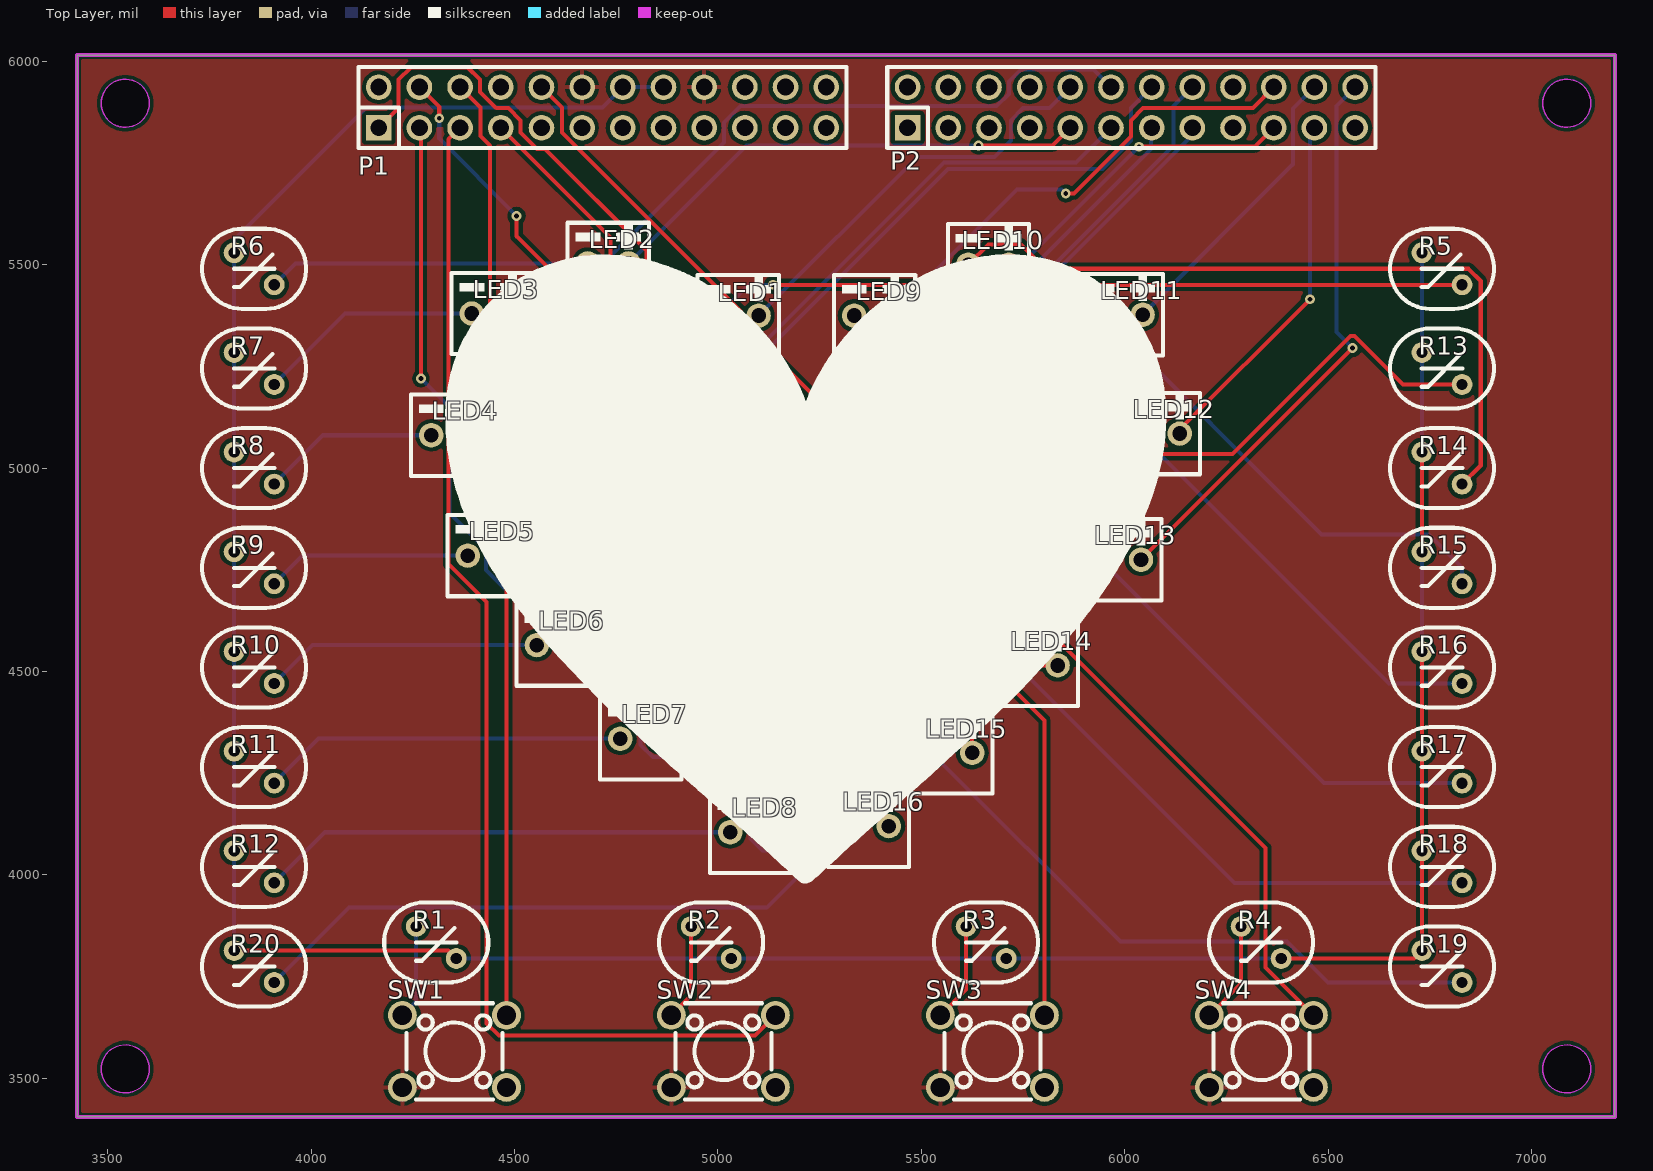
[diagram p0: Top Layer view]
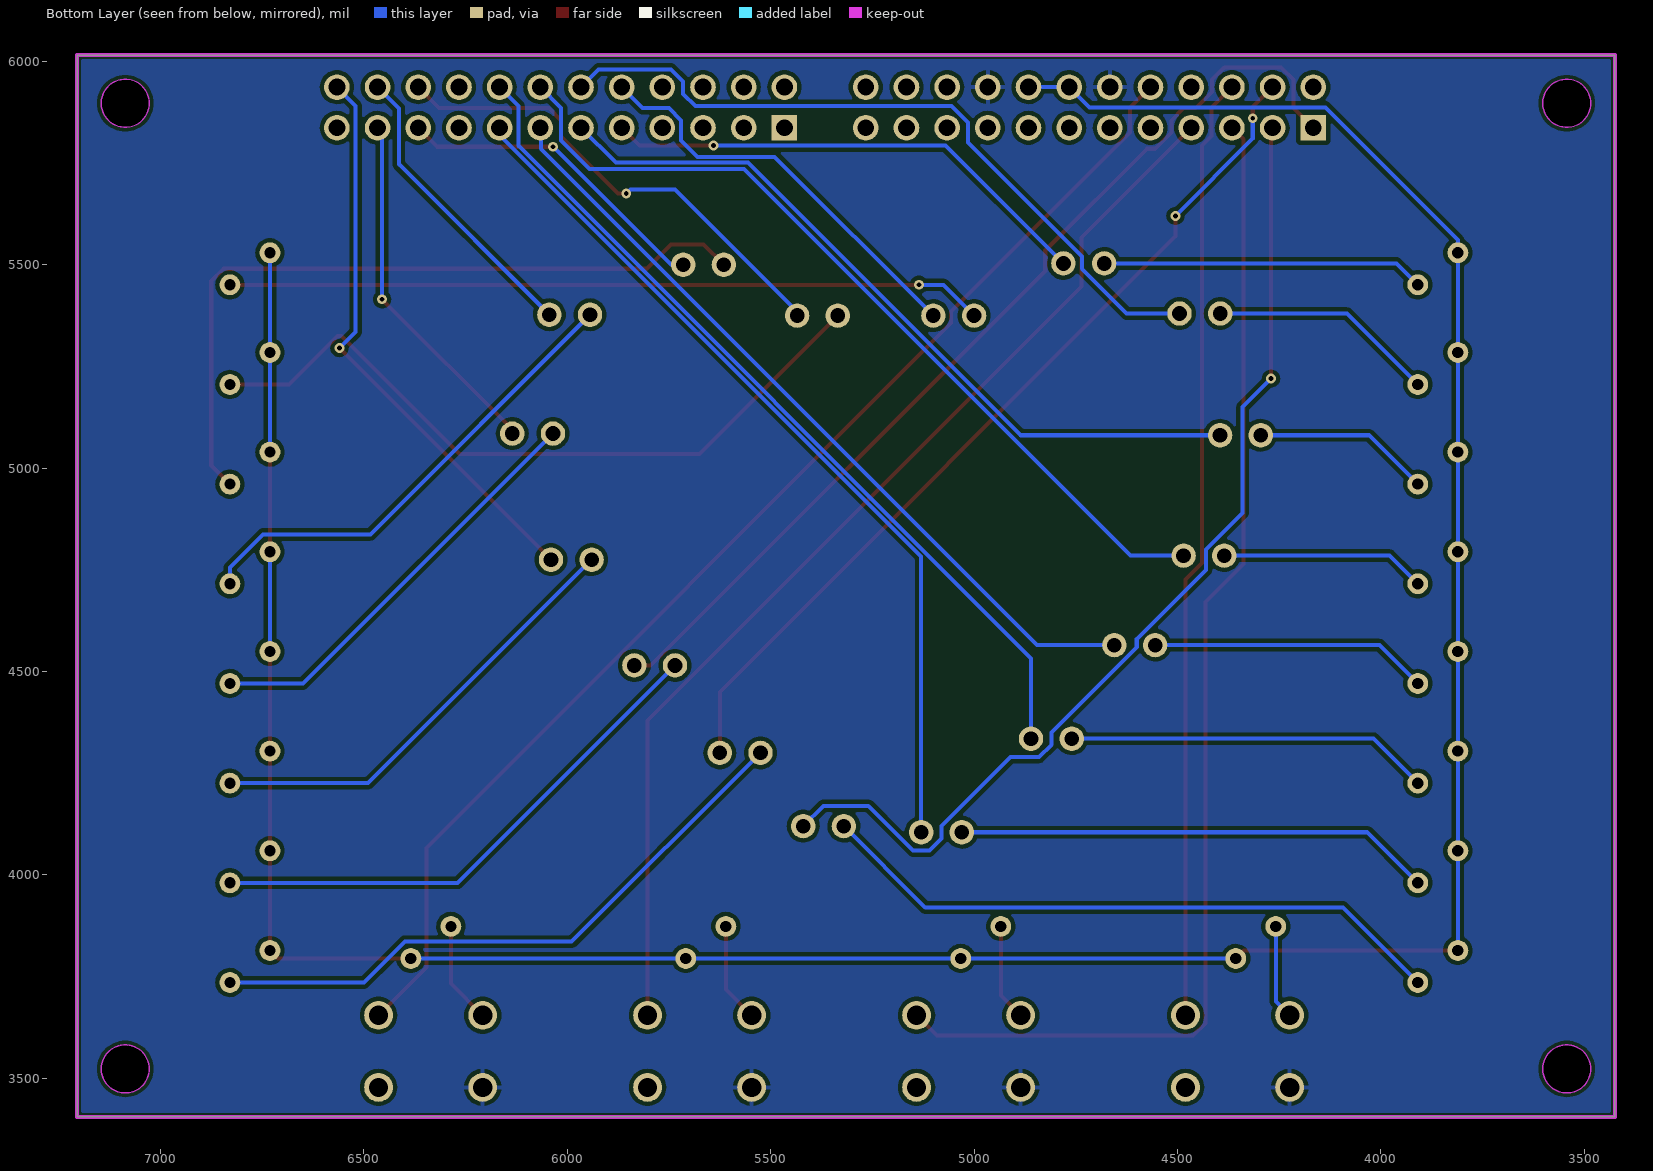
[diagram p1: Bottom Layer view, seen from below]
# Altium PCB MISC51818.pcbdoc
Units mil, origin at the board's own origin, x right, y up, seen from the top; angles counter-clockwise.
Board outline 3779.53 x 2609.84 mil, 2 copper layers (Top Layer, Bottom Layer), stack 62.206 mil thick; 42 components, 66 nets, 136 pads, 9 vias.

## Layer stack, top to bottom
Top Solder Mask Layer: solder mask 0.394, Dk 3.3
Top Layer: signal copper 1.379
Dielectric1: surface 59.449, FR4, Dk 4.5
Bottom Layer: signal copper 1.378
Bottom Solder Mask Layer: solder mask 0.394, Dk 3.3

## Board outline
3425,6015 3425,3405.16 7204.53,3405.16 7204.53,6015
cut-out: 3602.17,5896.89 cw(c3543.11,5896.89) 3484.06,5896.89 cw(c3543.11,5896.89)
cut-out: 3602.17,3523.27 cw(c3543.11,3523.27) 3484.06,3523.27 cw(c3543.11,3523.27)
cut-out: 7145.47,3523.27 cw(c7086.42,3523.27) 7027.36,3523.27 cw(c7086.42,3523.27)
cut-out: 7145.47,5896.89 cw(c7086.42,5896.89) 7027.36,5896.89 cw(c7086.42,5896.89)

## Design rules (kind name [scope] priority, off if disabled: settings)
BoardOutlineClearance copperThickness2oz_1 [All] p2 off: genericclearance=7.99 ignorepadtopadclearanceinfootprint=FALSE except(0: Arc-SplitContinuation Track-SplitContinuation SMDPad-SplitContinuation THPad-SplitContinuation Via-SplitContinuation Fill-SplitContinuation Region-SplitContinuation Poly-SplitContinuation Text-SplitContinuation Hole-SplitContinuation; 5.98: Arc-CutoutEdge SMDPad-CutoutEdge THPad-CutoutEdge Via-CutoutEdge Fill-CutoutEdge Region-CutoutEdge Text-CutoutEdge; 6.93: Hole-OutlineEdge Hole-CutoutEdge; 10: Poly-OutlineEdge Poly-CutoutEdge; 11.81: Arc-OutlineEdge Track-OutlineEdge SMDPad-OutlineEdge THPad-OutlineEdge Via-OutlineEdge Fill-OutlineEdge Region-OutlineEdge Text-OutlineEdge Track-CutoutEdge)
BoardOutlineClearance Plane_innerPlane_1 [All] p4 off: genericclearance=4.02 ignorepadtopadclearanceinfootprint=FALSE except(0: Arc-SplitContinuation Track-SplitContinuation SMDPad-SplitContinuation THPad-SplitContinuation Via-SplitContinuation Fill-SplitContinuation Region-SplitContinuation Poly-SplitContinuation Text-SplitContinuation Hole-SplitContinuation; 6: SMDPad-CutoutEdge THPad-CutoutEdge Via-CutoutEdge Fill-CutoutEdge Region-CutoutEdge Text-CutoutEdge; 6.93: Hole-OutlineEdge Hole-CutoutEdge; 10: Poly-OutlineEdge Poly-CutoutEdge; 11.8: Arc-OutlineEdge Track-OutlineEdge SMDPad-OutlineEdge THPad-OutlineEdge Via-OutlineEdge Fill-OutlineEdge Region-OutlineEdge Text-OutlineEdge; 11.81: Arc-CutoutEdge Track-CutoutEdge)
BoardOutlineClearance Copper_copperRegion_1 [All] p6 off: genericclearance=4.02 ignorepadtopadclearanceinfootprint=FALSE except(0: Arc-SplitContinuation Track-SplitContinuation SMDPad-SplitContinuation THPad-SplitContinuation Via-SplitContinuation Fill-SplitContinuation Region-SplitContinuation Poly-SplitContinuation Text-SplitContinuation Hole-SplitContinuation; 6: SMDPad-CutoutEdge THPad-CutoutEdge Via-CutoutEdge Fill-CutoutEdge Region-CutoutEdge Text-CutoutEdge; 6.93: Hole-OutlineEdge Hole-CutoutEdge; 10: Poly-OutlineEdge Poly-CutoutEdge; 11.8: Arc-OutlineEdge Track-OutlineEdge SMDPad-OutlineEdge THPad-OutlineEdge Via-OutlineEdge Fill-OutlineEdge Region-OutlineEdge Text-OutlineEdge; 11.81: Arc-CutoutEdge Track-CutoutEdge)
BoardOutlineClearance copperThickness1oz_1 [All] p8: genericclearance=4.02 ignorepadtopadclearanceinfootprint=FALSE except(0: Arc-SplitContinuation Track-SplitContinuation SMDPad-SplitContinuation THPad-SplitContinuation Via-SplitContinuation Fill-SplitContinuation Region-SplitContinuation Poly-SplitContinuation Text-SplitContinuation Hole-SplitContinuation; 6: SMDPad-CutoutEdge THPad-CutoutEdge Via-CutoutEdge Fill-CutoutEdge Region-CutoutEdge Text-CutoutEdge; 6.93: Hole-OutlineEdge Hole-CutoutEdge; 10: Poly-OutlineEdge Poly-CutoutEdge; 11.8: Arc-OutlineEdge Track-OutlineEdge SMDPad-OutlineEdge THPad-OutlineEdge Via-OutlineEdge Fill-OutlineEdge Region-OutlineEdge Text-OutlineEdge; 11.81: Arc-CutoutEdge Track-CutoutEdge)
Clearance copperThickness2oz [All] p1 off: gap=7.99 ignorepadtopadclearanceinfootprint=FALSE except(5.98: SMDPad-Track SMDPad-SMDPad THPad-Track SMDPad-THPad THPad-THPad Track-Via SMDPad-Via THPad-Via Via-Via Fill-Track Region-Track Fill-SMDPad Region-SMDPad Fill-THPad Region-THPad Fill-Via Region-Via Fill-Fill Fill-Region Region-Region Arc-Track Arc-SMDPad Arc-THPad Arc-Via Fill-Arc Region-Arc Arc-Arc Text-Track SMDPad-Text Text-THPad Text-Via Fill-Text Region-Text Arc-Text Text-Text; 6.93: Hole-Track Hole-SMDPad Hole-THPad Hole-Via Fill-Hole Region-Hole Hole-Arc Hole-Text; 10: Poly-Track Poly-SMDPad Poly-THPad Poly-Via Poly-Fill Poly-Region Poly-Poly Poly-Arc Poly-Text Poly-Hole)
Clearance Plane_innerPlane [All] p3 off: gap=4.02 ignorepadtopadclearanceinfootprint=FALSE except(5.98: SMDPad-Track SMDPad-SMDPad THPad-Track SMDPad-THPad THPad-THPad Track-Via SMDPad-Via THPad-Via Via-Via Fill-Track Region-Track Fill-SMDPad Region-SMDPad Fill-THPad Region-THPad Fill-Via Region-Via Fill-Fill Fill-Region Region-Region; 6: Arc-Track Arc-SMDPad Arc-THPad Arc-Via Fill-Arc Region-Arc Arc-Arc Text-Track SMDPad-Text Text-THPad Text-Via Fill-Text Region-Text Arc-Text Text-Text; 6.93: Hole-Track Hole-SMDPad Hole-THPad Hole-Via Fill-Hole Region-Hole Hole-Arc Hole-Text; 10: Poly-Track Poly-SMDPad Poly-THPad Poly-Via Poly-Fill Poly-Region Poly-Poly Poly-Arc Poly-Text Poly-Hole)
Clearance Copper_copperRegion [All] p5 off: gap=4.02 ignorepadtopadclearanceinfootprint=FALSE except(5.98: SMDPad-Track SMDPad-SMDPad THPad-Track SMDPad-THPad THPad-THPad Track-Via SMDPad-Via THPad-Via Via-Via Fill-Track Region-Track Fill-SMDPad Region-SMDPad Fill-THPad Region-THPad Fill-Via Region-Via Fill-Fill Fill-Region Region-Region; 6: Arc-Track Arc-SMDPad Arc-THPad Arc-Via Fill-Arc Region-Arc Arc-Arc Text-Track SMDPad-Text Text-THPad Text-Via Fill-Text Region-Text Arc-Text Text-Text; 6.93: Hole-Track Hole-SMDPad Hole-THPad Hole-Via Fill-Hole Region-Hole Hole-Arc Hole-Text; 10: Poly-Track Poly-SMDPad Poly-THPad Poly-Via Poly-Fill Poly-Region Poly-Poly Poly-Arc Poly-Text Poly-Hole)
Clearance copperThickness1oz [All] p7: gap=4.02 ignorepadtopadclearanceinfootprint=FALSE except(5.98: SMDPad-Track SMDPad-SMDPad THPad-Track SMDPad-THPad THPad-THPad Track-Via SMDPad-Via THPad-Via Via-Via Fill-Track Region-Track Fill-SMDPad Region-SMDPad Fill-THPad Region-THPad Fill-Via Region-Via Fill-Fill Fill-Region Region-Region; 6: Arc-Track Arc-SMDPad Arc-THPad Arc-Via Fill-Arc Region-Arc Arc-Arc Text-Track SMDPad-Text Text-THPad Text-Via Fill-Text Region-Text Arc-Text Text-Text; 6.93: Hole-Track Hole-SMDPad Hole-THPad Hole-Via Fill-Hole Region-Hole Hole-Arc Hole-Text; 10: Poly-Track Poly-SMDPad Poly-THPad Poly-Via Poly-Fill Poly-Region Poly-Poly Poly-Arc Poly-Text Poly-Hole)
DiffPairsRouting differentialPair [All] p1: maxlimit=6 minlimit=6 mostfreqgap=6 toplayer_minwidth=5 toplayer_prefwidth=10 toplayer_maxwidth=100 toplayer_mingap=6 toplayer_prefgap=6 toplayer_maxgap=6 bottomlayer_minwidth=5 bottomlayer_prefwidth=10 bottomlayer_maxwidth=100 bottomlayer_mingap=6 bottomlayer_prefgap=6 bottomlayer_maxgap=6 maxuncoupledlength=10
HoleToHoleClearance otherClearance [All] p1: gap=11.81 allowstackedmicrovias=TRUE
Length netLength [All] p1: minlimit=0 maxlimit=0
PasteMaskExpansion pasteMaskExpansion [All] p1: expansion=0
PlaneConnect innerPlane [All] p1: planeconnectstyle=Relief reliefexpansion=20 reliefentries=4 reliefconductorwidth=10 reliefairgap=10
PolygonConnect copperRegion [All] p1: connectstyle=Relief reliefconductorwidth=10 reliefentries=4 polygonreliefangle="90 Angle" airgapwidth=10 via.connectstyle=Relief via.reliefconductorwidth=10 via.reliefentries=4 via.polygonreliefangle="90 Angle" via.airgapwidth=10
RoutingVias viaSize [All] p1: holewidth=12.01 width=24.02 viastyle="Through Hole" minholewidth=11.81 minwidth=19.68 maxholewidth=248.03 maxwidth=393.7
SolderMaskExpansion solderMaskExpansion [IsVia] p1: expansion=-1000 istentingtop=TRUE
SolderMaskExpansion solderMaskExpansion [All] p2: expansion=2 istentingtop=FALSE
Width copperThickness2oz_2 [All] p1 off: maxlimit=100 minlimit=8 preferedwidth=10
Width copperThickness1oz_2 [All] p2: maxlimit=100 minlimit=5 preferedwidth=10

## Components (designator, comment, footprint, x,y, rotation, side; value= is the part's Value field where it differs from the comment)
LED1 "" LED-TH_L5.0-W5.0-P2.54_RED 5050,5375 r180 top
LED2 "" LED-TH_L5.0-W5.0-P2.54_RED 4730.3,5503.15 r180 top
LED3 "" LED-TH_L5.0-W5.0-P2.54_RED 4445,5380 r180 top
LED4 "" LED-TH_L5.0-W5.0-P2.54_RED 4345.3,5080.86 r180 top
LED5 "" LED-TH_L5.0-W5.0-P2.54_RED 4435,4785 r180 top
LED6 "" LED-TH_L5.0-W5.0-P2.54_RED 4605,4565 r180 top
LED7 "" LED-TH_L5.0-W5.0-P2.54_RED 4810,4335 r180 top
LED8 "" LED-TH_L5.0-W5.0-P2.54_RED 5080,4105 r180 top
LED9 "" LED-TH_L5.0-W5.0-P2.54_RED 5385,5375 r180 top
LED10 "" LED-TH_L5.0-W5.0-P2.54_RED 5665,5500 r180 top
LED11 "" LED-TH_L5.0-W5.0-P2.54_RED 5993.93,5377 r180 top
LED12 "" LED-TH_L5.0-W5.0-P2.54_RED 6085,5085 r180 top
LED13 "" LED-TH_L5.0-W5.0-P2.54_RED 5990,4775 r180 top
LED14 "" LED-TH_L5.0-W5.0-P2.54_RED 5785,4515 r180 top
LED15 "" LED-TH_L5.0-W5.0-P2.54_RED 5575,4300 r180 top
LED16 "" LED-TH_L5.0-W5.0-P2.54_RED 5370,4120 r180 top
P1 "2.54-2*12P female" HDR-TH_24P-P2.54-V-F-R2-C12-S2.54 4716.19,5886.46 r0 top
P2 "2.54-2*12P female" HDR-TH_24P-P2.54-V-F-R2-C12-S2.54 6016.19,5886.46 r0 top
R1 "4.7K" RES-TH_RES-TH_L6.5-W5.0-P2.50-D0.4-S2.00 4307.53,3834.14 r0 top
R2 "4.7K" RES-TH_RES-TH_L6.5-W5.0-P2.50-D0.4-S2.00 4983.42,3834.14 r0 top
R3 "4.7K" RES-TH_RES-TH_L6.5-W5.0-P2.50-D0.4-S2.00 5659.31,3834.14 r0 top
R4 "4.7K" RES-TH_RES-TH_L6.5-W5.0-P2.50-D0.4-S2.00 6335.2,3834.14 r0 top
R5 "1K" RES-TH_RES-TH_L6.5-W5.0-P2.50-D0.4-S2.00 6780,5490 r0 top
R6 "1K" RES-TH_RES-TH_L6.5-W5.0-P2.50-D0.4-S2.00 3860,5490 r0 top
R7 "1K" RES-TH_RES-TH_L6.5-W5.0-P2.50-D0.4-S2.00 3860,5245 r0 top
R8 "1K" RES-TH_RES-TH_L6.5-W5.0-P2.50-D0.4-S2.00 3860,5000 r0 top
R9 "1K" RES-TH_RES-TH_L6.5-W5.0-P2.50-D0.4-S2.00 3860,4755 r0 top
R10 "1K" RES-TH_RES-TH_L6.5-W5.0-P2.50-D0.4-S2.00 3860,4510 r0 top
R11 "1K" RES-TH_RES-TH_L6.5-W5.0-P2.50-D0.4-S2.00 3860,4265 r0 top
R12 "1K" RES-TH_RES-TH_L6.5-W5.0-P2.50-D0.4-S2.00 3860,4020 r0 top
R13 "1K" RES-TH_RES-TH_L6.5-W5.0-P2.50-D0.4-S2.00 6780,5245 r0 top
R14 "1K" RES-TH_RES-TH_L6.5-W5.0-P2.50-D0.4-S2.00 6780,5000 r0 top
R15 "1K" RES-TH_RES-TH_L6.5-W5.0-P2.50-D0.4-S2.00 6780,4755 r0 top
R16 "1K" RES-TH_RES-TH_L6.5-W5.0-P2.50-D0.4-S2.00 6780,4510 r0 top
R17 "1K" RES-TH_RES-TH_L6.5-W5.0-P2.50-D0.4-S2.00 6780,4265 r0 top
R18 "1K" RES-TH_RES-TH_L6.5-W5.0-P2.50-D0.4-S2.00 6780,4020 r0 top
R19 "1K" RES-TH_RES-TH_L6.5-W5.0-P2.50-D0.4-S2.00 6780,3775 r0 top
R20 "1K" RES-TH_RES-TH_L6.5-W5.0-P2.50-D0.4-S2.00 3860,3775 r0 top
SW1 "TS665CJ" SW-TH_4P-L6.0-W6.0-P4.50-LS6.5 4352.21,3566.44 r0 top
SW2 "TS665CJ" SW-TH_4P-L6.0-W6.0-P4.50-LS6.5 5013.41,3566.44 r0 top
SW3 "TS665CJ" SW-TH_4P-L6.0-W6.0-P4.50-LS6.5 5674.6,3566.44 r0 top
SW4 "TS665CJ" SW-TH_4P-L6.0-W6.0-P4.50-LS6.5 6335.8,3566.44 r0 top

## Footprints (in the part's own frame and the unit in brackets; to place one, negate y for a bottom-side part, rotate by r counter-clockwise, add the part's x,y. Pads: shape width x height; smd on the part's side, far side on the other; paste and mask are expansions set on the pad)
HDR-TH_24P-P2.54-V-F-R2-C12-S2.54 [mm]
  rect 1.6x1.6 hole 1.05: 1(-13.97,-1.27)
  round 1.6 hole 1.05: 2(-13.97,1.27) 3(-11.43,-1.27) 4(-11.43,1.27) 5(-8.89,-1.27) 6(-8.89,1.27) 7(-6.35,-1.27) 8(-6.35,1.27) 9(-3.81,-1.27) 10(-3.81,1.27) 11(-1.27,-1.27) 12(-1.27,1.27) 13(1.27,-1.27) 14(1.27,1.27) 15(3.81,-1.27) 16(3.81,1.27) 17(6.35,-1.27) 18(6.35,1.27) 19(8.89,-1.27) 20(8.89,1.27) 21(11.43,-1.27) 22(11.43,1.27) 23(13.97,-1.27) 24(13.97,1.27)
  silkscreen extent -15.24,-2.54 15.24,2.54
LED-TH_L5.0-W5.0-P2.54_RED [mil]
  round 60 hole 36 paste+0 mask+1.97: 1(-50,0) 2(50,0)
  silkscreen extent -100,-100 100,100
RES-TH_RES-TH_L6.5-W5.0-P2.50-D0.4-S2.00 [mm]
  round 1.3 hole 0.7: 1(-1.25,1) 2(1.25,-1)
  silkscreen extent -3.25,-2.5 3.25,2.5
SW-TH_4P-L6.0-W6.0-P4.50-LS6.5 [mm]
  round 1.8 hole 1.2: 1(-3.25,2.25) 2(3.25,2.25) 3(-3.25,-2.25) 4(3.25,-2.25)
  silkscreen extent -3,-3 3,3

## Via types
v1: diameter 24.02, hole 12, Top Layer to Bottom Layer, 9 vias

## Nets (pads, with @x,y where several pads share a name; then routed paths per layer and width w, separated by ;. In a path a pad name is that pad's centre, name@x,y a point inside that pad or via, vN(x,y) a via of type N, cw(c..) or ccw(c..) an arc to the next point about the centre after c; other vN are vias at no path point)
$1N1: R1.1 SW1.1 | length 232.6
  Bottom Layer w10: SW1.1 4258.32,3689.07 R1.1
$1N8: R2.1 SW2.1 | length 238.7
  Top Layer w10: SW2.1 4934.21,3703.77 R2.1
$1N12: R3.1 SW3.1 | length 244.8
  Top Layer w10: SW3.1 5610.1,3718.46 R3.1
$1N16: R4.1 SW4.1 | length 250.9
  Top Layer w10: SW4.1@6207.86,3655.01 6285.99,3733.15 R4.1
$1N17: LED1.2 R5.2 | length 1860.5
  Top Layer w10: v1(5135.63,5450.63) R5.2
  Bottom Layer w10: LED1.2 5075.63,5450.63 v1(5135.63,5450.63)
$1N18: LED2.2 R6.2 | length 792.8
  Bottom Layer w10: R6.2 3961.73,5503.15 LED2.2
$1N19: LED3.2 R7.2 | length 558
  Bottom Layer w10: R7.2 4083.58,5380 LED3.2
$1N20: LED4.2 R8.2 | length 435.9
  Bottom Layer w10: R8.2 4029.44,5080.86 LED4.2
$1N21: LED5.2 R9.2 | length 504.5
  Bottom Layer w10: R9.2 3978.58,4785 LED5.2
$1N22: LED8.2 R12.2 | length 1172.3
  Bottom Layer w10: R12.2 4033.58,4105 LED8.2
$1N23: LED6.2 R10.2 | length 684.9
  Bottom Layer w10: R10.2 4003.58,4565 LED6.2
$1N24: LED7.2 R11.2 | length 896.1
  Bottom Layer w10: R11.2 4018.58,4335 LED7.2
$1N25: LED9.2 R13.2 | length 1804.6
  Top Layer w10: LED9.2 5675,5035 6265,5035 6555,5325 6565,5325 6684.37,5205.63 R13.2
$1N26: LED13.2 R17.2 | length 1116.8
  Bottom Layer w10: LED13.2 6489.37,4225.63 R17.2
$1N27: LED12.2 R16.2 | length 1048.7
  Bottom Layer w10: LED12.2 6649.37,4470.63 R16.2
$1N28: LED11.2 R15.2 | length 1182.7
  Bottom Layer w10: LED11.2 6483.93,4837 6747.84,4837 6829.21,4755.63 R15.2
$1N29: LED14.2 R18.2 | length 1315.6
  Bottom Layer w10: LED14.2 6269.37,3980.63 R18.2
$1N30: LED10.2 R14.2 | length 1836.3
  Top Layer w10: LED10.2 5665,5550 5745,5550 5805,5490 6845,5490 6875,5460 6875,5006.41 R14.2
$1N31: LED16.2 R20.2 | length 1570
  Bottom Layer w10: R20.2 4093.58,3920 5120,3920 LED16.2
$1N32: LED15.2 R19.2 | length 1538
  Bottom Layer w10: LED15.2 5989.01,3835.99 6399.01,3835.99 6499.37,3735.63 R19.2
GND: P1.12 P1.18 SW1.3 SW2.3 SW3.3 SW4.3
P00: LED9.1 P2.20 | length 1201.3
  Top Layer w10: v1(5855,5675) 5875,5675 6015,5815 6015,5855 6045,5885 6314.72,5885 P2.20
  Bottom Layer w10: LED9.1 5435,5385 5735,5685 5845,5685 v1(5855,5675)
P01: LED10.1 P2.19 | length 790.6
  Top Layer w10: v1(6035,5790) 6319.72,5790 P2.19
  Bottom Layer w10: LED10.1 5745,5500 v1(6035,5790)
P02: LED11.1 P2.22 | length 734.4
  Bottom Layer w10: LED11.1 6413.93,5747 6413.93,5884.2 P2.22
P03: LED12.1 P2.21 | length 888.6
  Top Layer w10: LED12.1 6135,5095 v1(6455,5415)
  Bottom Layer w10: v1(6455,5415) 6455,5825.28 P2.21
P04: LED13.1 P2.24 | length 1412.6
  Top Layer w10: LED13.1 v1(6560,5295)
  Bottom Layer w10: v1(6560,5295) 6520,5335 6520,5890.28 P2.24
P05: LED14.1 P1.1 | length 2444.5
  Top Layer w10: P1.1 4215,5885.28 4215,5955 4245,5985 4385,5985 4415,5955 4415,5925 4455,5885 4485,5885 4515,5855 4515,5825 4555,5785 4575,5785 4825,5535 4825,5485 5795,4515 LED14.1
P06: LED15.1 P1.4 | length 2199.3
  Top Layer w10: P1.4 4315,5887.65 v1(4315,5860) ; v1(4505,5620) 4505,5570 5625,4450 LED15.1
  Bottom Layer w10: v1(4315,5860) 4315,5810 v1(4505,5620)
P07: LED16.1 P1.3 | length 2543.3
  Top Layer w10: P1.3 4270,5832.65 v1(4270,5220)
  Bottom Layer w10: v1(4270,5220) 4340,5150 4340,4890 4430,4800 4430,4750 4600,4580 4600,4560 4810,4350 4810,4320 4840,4290 4910,4290 5080,4120 5080,4090 5110,4060 5150,4060 5260,4170 5370,4170 LED16.1
P10: P1.6 SW1.2 | length 2328.7
  Top Layer w10: P1.6 4416.19,5886.46 4416.19,5816.46 4440.16,5792.49 4440.16,4766.46 4480.16,4726.47 SW1.2
P11: P1.5 SW2.2 | length 2994.8
  Top Layer w10: P1.5 4338.19,5808.47 4338.19,4764.46 4431.36,4671.3 4431.36,3635.01 4461.36,3605.01 5091.35,3605.01 SW2.2
P12: P1.7 SW3.2 | length 2735
  Top Layer w10: P1.7 4736.19,5566.46 4736.19,5446.46 5802.55,4380.1 SW3.2
P16: P1.10 SW4.2 | length 3067.4
  Top Layer w10: P1.10 4616.19,5886.46 4616.19,5825.1 5056.18,5385.11 5056.18,5356.46 6346.18,4066.47 6346.18,3772.59 SW4.2
P17: P1.9
P20: LED1.1 P2.10 | length 1028
  Bottom Layer w10: LED1.1 5490,5765 5680,5765 5720,5805 5720,5855 5750,5885 5814.72,5885 P2.10
P21: LED2.1 P2.9 | length 1224
  Top Layer w10: v1(5640.29,5793.15) 5822.87,5793.15 P2.9
  Bottom Layer w10: LED2.1 5070.3,5793.15 v1(5640.29,5793.15)
P22: LED3.1 P2.12 | length 1802.2
  Bottom Layer w10: LED3.1 4625,5380 4735,5490 4735,5520 5015,5800 5015,5850 5055,5890 5685,5890 5715,5920 5715,5950 5745,5980 5922.65,5980 P2.12
P23: LED4.1 P2.11 | length 1883.9
  Bottom Layer w10: LED4.1 4885.3,5080.86 5555.29,5750.86 5880.58,5750.86 P2.11
P24: LED5.1 P2.14 | length 2105.2
  Bottom Layer w10: LED5.1 4615,4785 5565,5735 5945,5735 6015,5805 6015,5885.27 P2.14
P25: LED6.1 P2.13 | length 1967.3
  Bottom Layer w10: LED6.1 4845,4565 6065,5785 6065,5835.27 P2.13
P26: LED7.1 P2.16 | length 2142.5
  Bottom Layer w10: LED7.1 4860,4532.48 6120,5792.48 6120,5890.27 P2.16
P27: LED8.1 P2.15 | length 2160.7
  Bottom Layer w10: LED8.1 5130,4782.48 6166.19,5818.67 P2.15
P32: P1.22
P33: P1.21
P34: P1.24
P35: P2.1
P40: P1.17
P41: P2.6
P42: P2.5
P43: P2.8
P44: P2.7
P45: P2.18
P46: P2.17
P47: P1.8
P50: P1.23
P51: P2.2
P52: P2.23
P53: P1.2
P54: P1.13
P55: P1.15
RXD-1: P1.20
RXD-2: P2.4
TXD-1: P1.19
TXD-2: P2.3
VCC: P1.14 P1.16 R1.2 R2.2 R3.2 R4.2 R5.1 R6.1 R7.1 R8.1 R9.1 R10.1 R11.1 R12.1 R13.1 R14.1 R15.1 R16.1 R17.1 R18.1 R19.1 R20.1 | length 7608.8
  Top Layer w10: R20.1 4337.15,3814.37 R1.2 ; R4.2 6711.19,3794.77 R19.1 R18.1 R17.1 R16.1 ; R15.1 R14.1
  Bottom Layer w10: R20.1 R12.1 R11.1 R10.1 R9.1 R8.1 R7.1 R6.1 3810.79,5561.06 4136.19,5886.46 4716.19,5886.46 P1.14 P1.16 ; R1.2 R2.2 R3.2 R4.2 ; R16.1 R15.1 ; R14.1 R13.1 R5.1
VREF: P1.11
pads on no net: SW1.4 SW2.4 SW3.4 SW4.4

## Polygon pours and split planes (outlines as drawn)
GND on Top Layer (solid, remove dead copper, pour order 0): 3000,6240 3000,3000 7965,3000 7965,6240
GND on Bottom Layer (solid, remove dead copper, pour order 2): 3130,6250 3130,3175 7785,3175 7785,6250

## Keep-outs
Board Outline Layer:
  region: 3602.17,5896.89 cw(c3543.11,5896.89) 3484.06,5896.89 cw(c3543.11,5896.89)
  circle w0.1: c3543.11,5896.89 r59.06
  region: 3602.17,5896.89 3601.77,5890.03 3600.57,5883.27 3598.6,5876.69 3595.88,5870.39 3592.45,5864.44 3588.35,5858.93 3583.64,5853.93 3578.38,5849.52 3572.64,5845.75 3566.5,5842.66 3560.05,5840.32 3553.36,5838.73 3546.54,5837.93 3539.68,5837.93 3532.86,5838.73 3526.17,5840.32 3519.72,5842.66 3513.58,5845.75 3507.84,5849.52 3502.58,5853.93 3497.87,5858.93 3493.77,5864.44 3490.34,5870.39 3487.62,5876.69 3485.65,5883.27 3484.45,5890.03 3484.06,5896.89 3484.45,5903.75 3485.65,5910.51 3487.62,5917.09 3490.34,5923.39 3493.77,5929.34 3497.87,5934.85 3502.58,5939.84 3507.84,5944.26 3513.58,5948.03 3519.72,5951.12 3526.17,5953.46 3532.86,5955.05 3539.68,5955.85 3546.54,5955.85 3553.36,5955.05 3560.05,5953.46 3566.5,5951.12 3572.64,5948.03 3578.38,5944.26 3583.64,5939.84 3588.35,5934.85 3592.45,5929.34 3595.88,5923.39 3598.6,5917.09 3600.57,5910.51 3601.77,5903.75
  region: 3602.17,3523.27 cw(c3543.11,3523.27) 3484.06,3523.27 cw(c3543.11,3523.27)
  circle w0.1: c3543.11,3523.27 r59.06
  region: 3602.17,3523.27 3601.77,3516.41 3600.57,3509.65 3598.6,3503.07 3595.88,3496.76 3592.45,3490.82 3588.35,3485.31 3583.64,3480.31 3578.38,3475.9 3572.64,3472.12 3566.5,3469.04 3560.05,3466.69 3553.36,3465.11 3546.54,3464.31 3539.68,3464.31 3532.86,3465.11 3526.17,3466.69 3519.72,3469.04 3513.58,3472.12 3507.84,3475.9 3502.58,3480.31 3497.87,3485.31 3493.77,3490.82 3490.34,3496.76 3487.62,3503.07 3485.65,3509.65 3484.45,3516.41 3484.06,3523.27 3484.45,3530.12 3485.65,3536.89 3487.62,3543.47 3490.34,3549.77 3493.77,3555.72 3497.87,3561.23 3502.58,3566.22 3507.84,3570.64 3513.58,3574.41 3519.72,3577.49 3526.17,3579.84 3532.86,3581.43 3539.68,3582.22 3546.54,3582.22 3553.36,3581.43 3560.05,3579.84 3566.5,3577.49 3572.64,3574.41 3578.38,3570.64 3583.64,3566.22 3588.35,3561.23 3592.45,3555.72 3595.88,3549.77 3598.6,3543.47 3600.57,3536.89 3601.77,3530.12
  region: 7145.47,3523.27 cw(c7086.42,3523.27) 7027.36,3523.27 cw(c7086.42,3523.27)
  circle w0.1: c7086.42,3523.27 r59.06
  region: 7145.47,3523.27 7145.07,3516.41 7143.88,3509.65 7141.91,3503.07 7139.19,3496.76 7135.76,3490.82 7131.66,3485.31 7126.94,3480.31 7121.68,3475.9 7115.94,3472.12 7109.81,3469.04 7103.35,3466.69 7096.67,3465.11 7089.85,3464.31 7082.98,3464.31 7076.16,3465.11 7069.48,3466.69 7063.03,3469.04 7056.89,3472.12 7051.15,3475.9 7045.89,3480.31 7041.18,3485.31 7037.08,3490.82 7033.64,3496.76 7030.92,3503.07 7028.95,3509.65 7027.76,3516.41 7027.36,3523.27 7027.76,3530.12 7028.95,3536.89 7030.92,3543.47 7033.64,3549.77 7037.08,3555.72 7041.18,3561.23 7045.89,3566.22 7051.15,3570.64 7056.89,3574.41 7063.03,3577.49 7069.48,3579.84 7076.16,3581.43 7082.98,3582.22 7089.85,3582.22 7096.67,3581.43 7103.35,3579.84 7109.81,3577.49 7115.94,3574.41 7121.68,3570.64 7126.94,3566.22 7131.66,3561.23 7135.76,3555.72 7139.19,3549.77 7141.91,3543.47 7143.88,3536.89 7145.07,3530.12
  region: 7145.47,5896.89 cw(c7086.42,5896.89) 7027.36,5896.89 cw(c7086.42,5896.89)
  circle w0.1: c7086.42,5896.89 r59.06
  region: 7145.47,5896.89 7145.07,5890.03 7143.88,5883.27 7141.91,5876.69 7139.19,5870.39 7135.76,5864.44 7131.66,5858.93 7126.94,5853.93 7121.68,5849.52 7115.94,5845.75 7109.81,5842.66 7103.35,5840.32 7096.67,5838.73 7089.85,5837.93 7082.98,5837.93 7076.16,5838.73 7069.48,5840.32 7063.03,5842.66 7056.89,5845.75 7051.15,5849.52 7045.89,5853.93 7041.18,5858.93 7037.08,5864.44 7033.64,5870.39 7030.92,5876.69 7028.95,5883.27 7027.76,5890.03 7027.36,5896.89 7027.76,5903.75 7028.95,5910.51 7030.92,5917.09 7033.64,5923.39 7037.08,5929.34 7041.18,5934.85 7045.89,5939.84 7051.15,5944.26 7056.89,5948.03 7063.03,5951.12 7069.48,5953.46 7076.16,5955.05 7082.98,5955.85 7089.85,5955.85 7096.67,5955.05 7103.35,5953.46 7109.81,5951.12 7115.94,5948.03 7121.68,5944.26 7126.94,5939.84 7131.66,5934.85 7135.76,5929.34 7139.19,5923.39 7141.91,5917.09 7143.88,5910.51 7145.07,5903.75
  lines w10: 3425,3405.16 3425,6015 7204.53,6015 7204.53,3405.16 3425,3405.16

## Silkscreen, mask and mechanical layers (free items; w line width, h text height)
Top Silkscreen Layer:
  region: 569 vertices and 1 holes, not listed, extent 4330,3979.1 6101.65,5525
Mechanical Layer:
  circle w0.1: c3543.11,5896.89 r59.06
  circle w0.1: c3543.11,3523.27 r59.06
  circle w0.1: c7086.42,3523.27 r59.06
  circle w0.1: c7086.42,5896.89 r59.06

## Dimensions
5266.19,6072.66 to 5466.19,6072.66 on Document Layer
3425,6325 to 7204.53,6325 on Document Layer
7321.77,6015 to 7321.77,3405.16 on Document Layer
3425,6510 to 4173.45,6510 on Document Layer